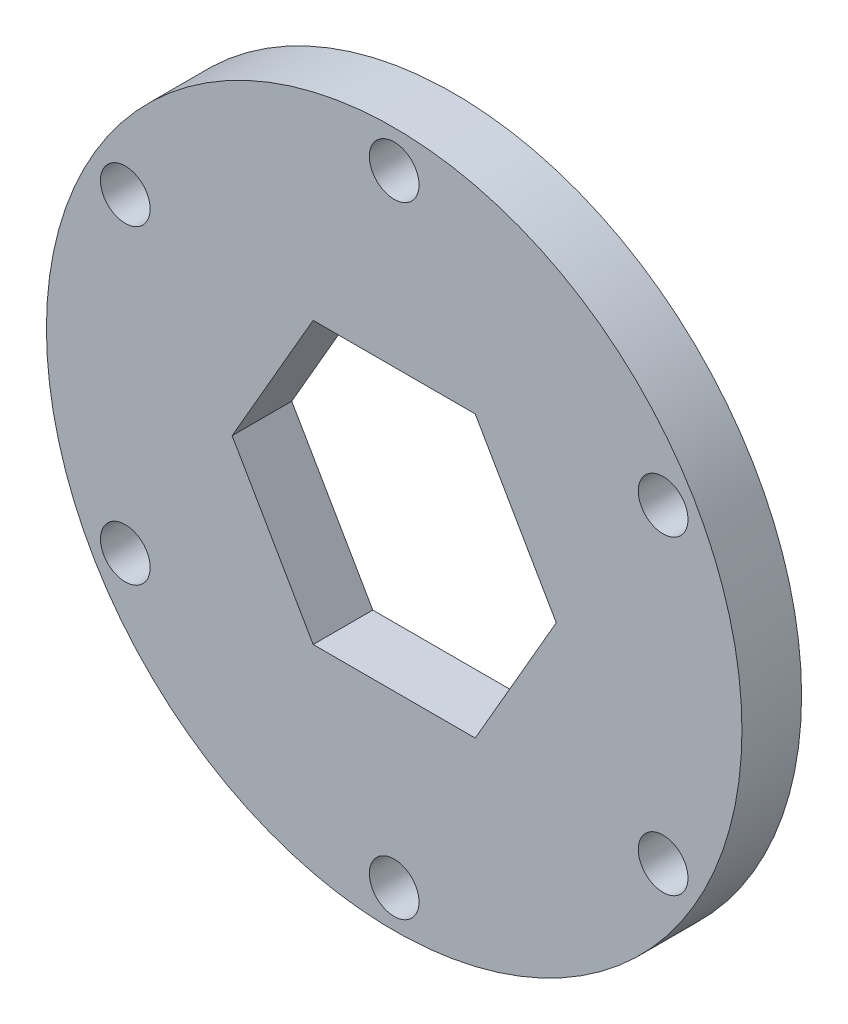
SolidWorks part; units mm, degrees
material "Q235B"
ref_plane "Front Plane" through (0, 0, 0) normal (0, 0, 1) x (1, 0, 0)
ref_plane "Top Plane" through (0, 0, 0) normal (0, 1, 0) x (1, 0, 0)
ref_plane "Right Plane" through (0, 0, 0) normal (1, 0, 0) x (0, 0, -1)
sketch "Sketch1" plane through (0, 0, 0) normal (0, 0, 1) x (1, 0, 0)
  line L1 (32.6203, 0) -> (16.3101, 28.25)
  line L2 (16.3101, 28.25) -> (-16.3101, 28.25)
  line L3 (-16.3101, 28.25) -> (-32.6203, 0)
  line L4 (-32.6203, 0) -> (-16.3101, -28.25)
  line L5 (-16.3101, -28.25) -> (16.3101, -28.25)
  line L6 (16.3101, -28.25) -> (32.6203, 0)
  circle A0 centre (0, 0) radius 70
  circle A1 centre (0, 0) radius 62.5 construction
  circle A2 centre (0, 62.5) radius 5
  circle A3 centre (54.1266, 31.25) radius 5
  circle A4 centre (54.1266, -31.25) radius 5
  circle A5 centre (0, -62.5) radius 5
  circle A6 centre (-54.1266, -31.25) radius 5
  circle A7 centre (-54.1266, 31.25) radius 5
  circle A8 centre (0, 0) radius 28.25 construction
  dimension "D1" = 140
  dimension "D2" = 125
  dimension "D3" = 10
  dimension "D5" = 56.5
  dimension "D4" = 6
extrude "Boss-Extrude1" add sketch "Sketch1" along normal blind 12
